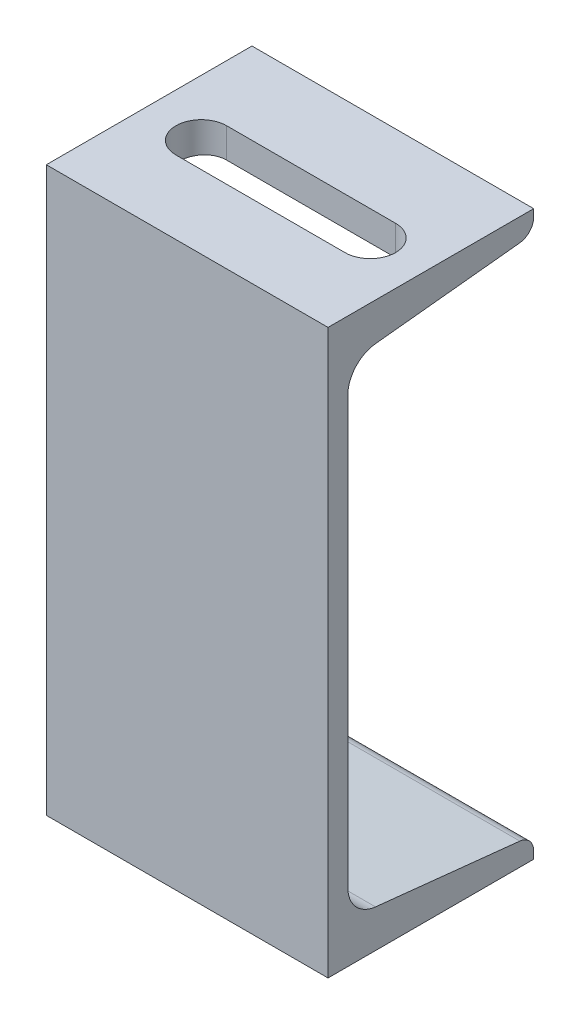
SolidWorks part; units mm, degrees
material "普通碳钢"
ref_plane "前视基准面" through (0, 0, 0) normal (0, 0, 1) x (1, 0, 0)
ref_plane "上视基准面" through (0, 0, 0) normal (0, 1, 0) x (1, 0, 0)
ref_plane "右视基准面" through (0, 0, 0) normal (1, 0, 0) x (0, 0, -1)
sketch3d "3D草图1"
  line L0 (0, 0, 0) -> (100, 0, 0)
  dimension "D1" = 100
other "C 槽 20A(1)"
ref_plane "基准面1" through (0, 0, 0) normal (1, 0, 0) x (0, 0, -1)
sketch "Sketch1" plane through (0, 0, 0) normal (1, 0, 0) x (0, 0, -1)
  line L0 (73, 200) -> (0, 200)
  line L1 (73, 0) -> (0, 0)
  line L2 (0, 200) -> (0, 0)
  line L3 (-9.5694, 100) -> (49.7414, 100) construction
  line L4 (7, 175.6271) -> (7, 24.3729)
  line L5 (73, 0) -> (73, 2.5793)
  line L6 (73, 200) -> (73, 197.4207)
  line L7 (16.8502, 13.4331) -> (68.0749, 8.0492)
  line L17 (16.8502, 186.5669) -> (68.0749, 191.9508)
  arc A0 (68.0749, 191.9508) -> (73, 197.4207) centre (67.5, 197.4207) ccw
  arc A1 (68.0749, 8.0492) -> (73, 2.5793) centre (67.5, 2.5793) cw
  arc A2 (7, 24.3729) -> (16.8502, 13.4331) centre (18, 24.3729) ccw
  arc A10 (7, 175.6271) -> (16.8502, 186.5669) centre (18, 175.6271) cw
  point P6 (0, 0)
  point P8 (0, 100)
  point P9 (7, 25.8841)
  point P10 (36.5, 200)
  point P13 (73, 192.4684)
  point P14 (40, 189)
  point P19 (7, 100)
sketch "草图2" plane through (0, 200, 0) normal (0, 1, 0) x (1, 0, 0)
  line L0 (20, 35) -> (80, 35) construction
  line L1 (20, 44) -> (80, 44)
  line L2 (20, 26) -> (80, 26)
  line L3 (100, 0) -> (0, 0) construction
  line L4 (0, 73) -> (0, 0) construction
  arc A0 (20, 44) -> (20, 26) centre (20, 35) ccw
  arc A1 (80, 26) -> (80, 44) centre (80, 35) ccw
  point P2 (50, 35)
  dimension "D1" = 35
  dimension "D2" = 60
  dimension "D3" = 20
  dimension "D4" = 18
extrude "切除-拉伸1" cut sketch "草图2" against normal blind 16
equation "\"RI@Sketch1\" = \"D1@Sketch1\""
equation "\"D3@Sketch1\" =  ( \"BF@Sketch1\" - \"D6@Sketch1\" )  / 2"
